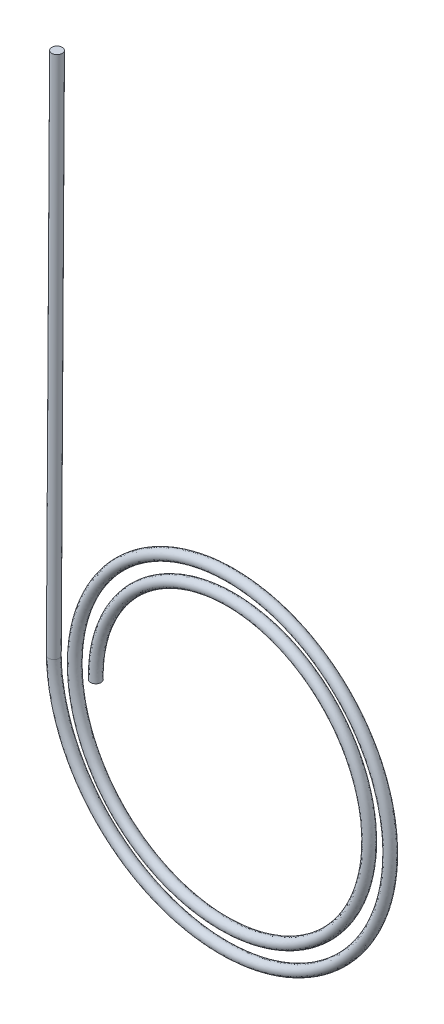
SolidWorks part; units mm, degrees
ref_plane "Front Plane" through (0, 0, 0) normal (0, 0, 1) x (1, 0, 0)
ref_plane "Top Plane" through (0, 0, 0) normal (0, 1, 0) x (1, 0, 0)
ref_plane "Right Plane" through (0, 0, 0) normal (1, 0, 0) x (0, 0, -1)
other "Configuration Table"
sketch "Sketch1" plane through (0, 0, 0) normal (0, 0, 1) x (1, 0, 0)
  circle A0 centre (0, 0) radius 12.5
  dimension "D1" = 25
curve "Helix/Spiral1"
sketch "Sketch2" plane through (0, 0, 0) normal (0, 1, 0) x (1, 0, 0)
  circle A0 centre (-12.5004, 0) radius 0.5
  dimension "D1" = 1
sweep "Sweep1" add profiles "Sketch2" path "Helix/Spiral1"
sketch "Sketch3" plane through (-0.0006, -0.1018, 0) normal (0.0062, 1, 0) x (1, -0.0062, 0)
  circle A0 centre (-16.5001, 0) radius 0.5
extrude "Boss-Extrude1" add sketch "Sketch3" along normal blind 50
sketch "Sketch4" plane through (0, 0, 0) normal (0, 0, 1) x (1, 0, 0)
  line L0 (-6.212, 0) -> (-6.212, 23.3258) construction
  circle A0 centre (0, 0) radius 6.212 construction
